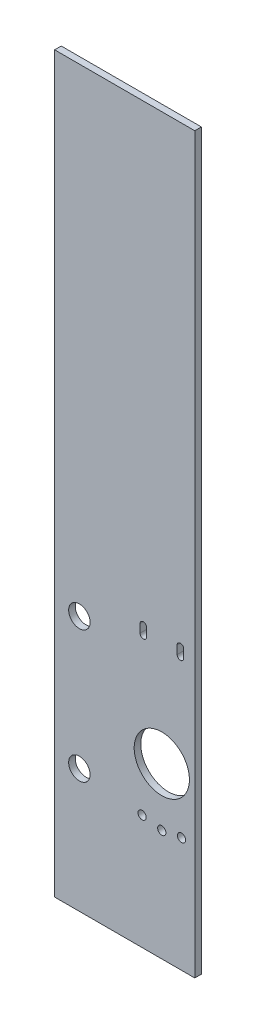
from build123d import *

# Parameters (mm, degrees)
SKETCH_1_W      = 85
SKETCH_1_H      = 445
SKETCH_1_R      = 6.5
SKETCH_1_R_2    = 2.5
SKETCH_1_R_3    = 16.75
EXTRUDE_2_DEPTH = 4


with BuildPart() as part:
    # 草图1 → 凸台-拉伸2 (new body)
    with BuildSketch(Plane.XY):
        with Locations((42.5, -222.5)):
            Rectangle(SKETCH_1_W, SKETCH_1_H)
        with Locations((15, -370)):
            Circle(SKETCH_1_R, mode=Mode.SUBTRACT)
        with Locations((76.970705016, -375.389241728)):
            Circle(SKETCH_1_R_2, mode=Mode.SUBTRACT)
        with Locations((65, -377.5)):
            Circle(SKETCH_1_R_2, mode=Mode.SUBTRACT)
        with Locations((15, -290)):
            Circle(SKETCH_1_R, mode=Mode.SUBTRACT)
        with Locations((53.029294983, -375.389241728)):
            Circle(SKETCH_1_R_2, mode=Mode.SUBTRACT)
        with Locations((65, -342.5)):
            Circle(SKETCH_1_R_3, mode=Mode.SUBTRACT)
        with BuildLine():
            Line((78.3, -275.5), (78.3, -280.5))
            ThreePointArc((78.3, -280.5), (76.3, -282.5), (74.3, -280.5))
            Line((74.3, -280.5), (74.3, -275.5))
            ThreePointArc((74.3, -275.5), (76.3, -273.5), (78.3, -275.5))
        make_face(mode=Mode.SUBTRACT)
        with BuildLine():
            Line((55.8, -275.5), (55.8, -280.5))
            ThreePointArc((55.8, -280.5), (53.8, -282.5), (51.8, -280.5))
            Line((51.8, -280.5), (51.8, -275.5))
            ThreePointArc((51.8, -275.5), (53.8, -273.5), (55.8, -275.5))
        make_face(mode=Mode.SUBTRACT)
    extrude(amount=EXTRUDE_2_DEPTH)


solid = part.part
